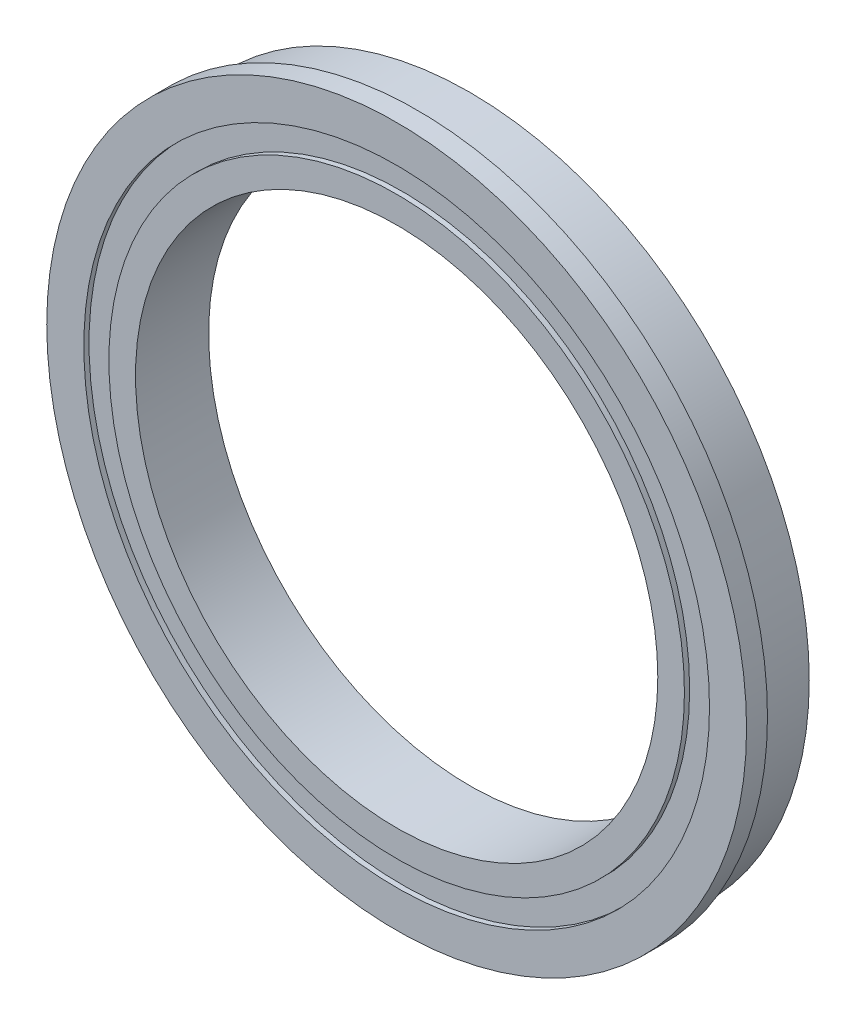
from build123d import *

# Parameters (mm, degrees)
EXTRUDE_START   = -2
SKETCH_2_R      = 33.5
SKETCH_2_R_2    = 32.5
EXTRUDE_1_DEPTH = 2


with BuildPart() as part:
    # 草图1 → 旋转1 (revolve)
    with BuildSketch(Plane(origin=(0, 0, 0), x_dir=(0, 0, -1), z_dir=(1, 0, 0)), mode=Mode.PRIVATE) as revolve_1_sk:
        Polygon((-3.5, 25), (-3.5, 27.55), (-3, 27.55), (-3, 29.95), (-3.5, 29.95), (-3.5, 32.5), (3.5, 32.5), (3.5, 29.95), (3, 29.95), (3, 27.55), (3.5, 27.55), (3.5, 25), align=None)
    revolve(revolve_1_sk.sketch.rotate(Axis((0, 0, 0), (0, 0, -1)), 90), axis=Axis((0, 0, 0), (0, 0, -1)))

    # 草图2 → 凸台-拉伸1 (add)
    with BuildSketch(Plane.XY.offset(3.5).offset(EXTRUDE_START)):
        Circle(SKETCH_2_R)
        Circle(SKETCH_2_R_2, mode=Mode.SUBTRACT)
    extrude(amount=EXTRUDE_1_DEPTH)


solid = part.part
